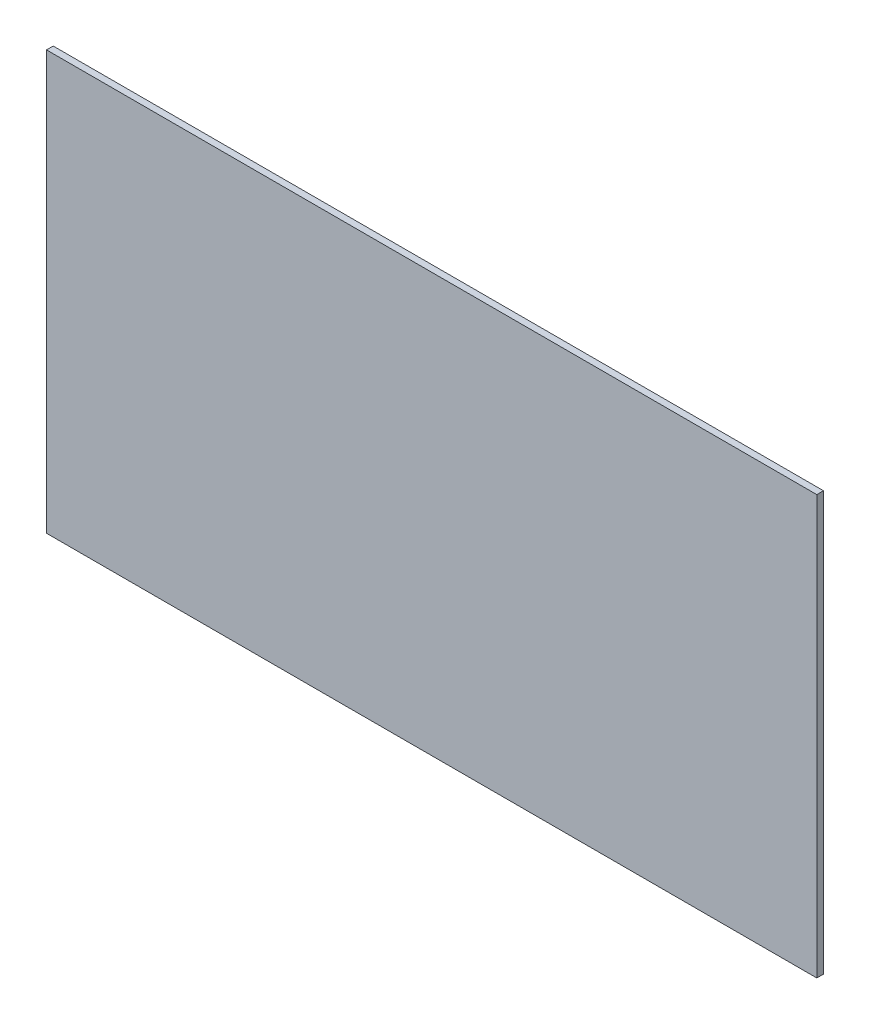
from build123d import *

# Parameters (mm, degrees)
SKETCH1_W           = 920
SKETCH1_H           = 500
BOSS_EXTRUDE1_DEPTH = 8


with BuildPart() as part:
    # Sketch1 → Boss-Extrude1 (new body)
    with BuildSketch(Plane.XY):
        Rectangle(SKETCH1_W, SKETCH1_H)
    extrude(amount=BOSS_EXTRUDE1_DEPTH)


solid = part.part
